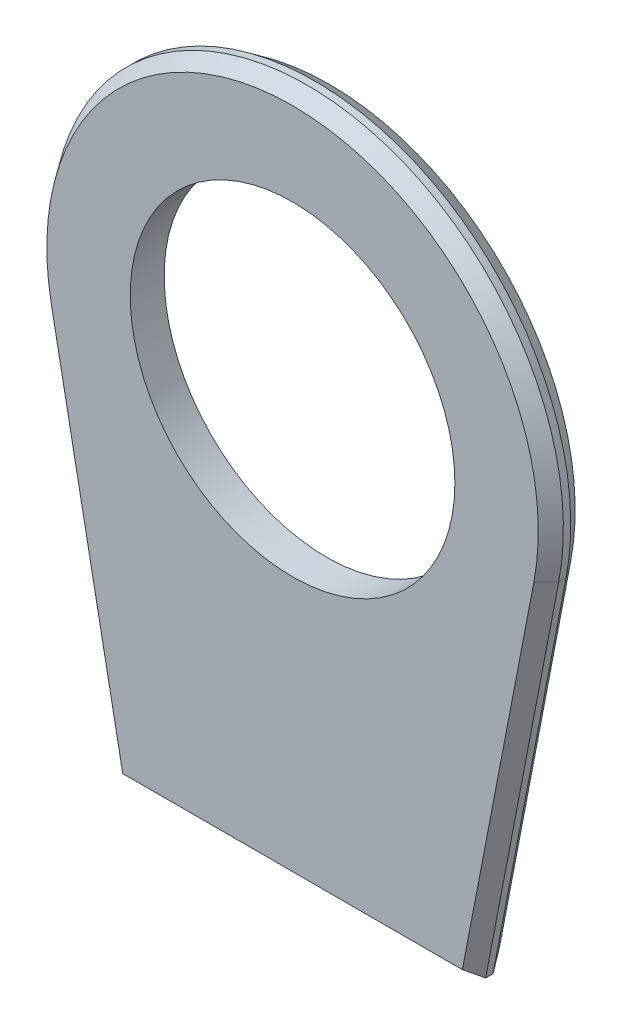
SolidWorks part; units mm, degrees
ref_plane "Front Plane" through (0, 0, 0) normal (0, 0, 1) x (1, 0, 0)
ref_plane "Top Plane" through (0, 0, 0) normal (0, 1, 0) x (1, 0, 0)
ref_plane "Right Plane" through (0, 0, 0) normal (1, 0, 0) x (0, 0, -1)
sketch "Sketch1" plane through (0, 0, 0) normal (0, 0, 1) x (1, 0, 0)
  line L0 (0, -94.8031) -> (0, 121.5186) construction
  line L1 (-120.85, 0) -> (120.85, 0)
  line L2 (120.85, 0) -> (170.3708, 257.1967)
  line L3 (-120.85, 0) -> (-170.3708, 257.1967)
  arc A0 (170.3708, 257.1967) -> (-170.3708, 257.1967) centre (0, 290) ccw
  circle A1 centre (0, 290) radius 110
  dimension "D1" = 347
  dimension "D5" = 220
  dimension "D2" = 290
  dimension "D3" = 241.7
  dimension "D4" = 241.7
extrude "Boss-Extrude1" add sketch "Sketch1" along normal blind 25
sketch "Sketch2" plane through (0, 0, 0) normal (0, 0, 1) x (1, 0, 0)
  circle A0 centre (0, 290) radius 110 construction
  circle A1 centre (0, 290) radius 110
  circle A2 centre (0, 290) radius 123
  dimension "D1" = 246
extrude "Cut-Extrude2" cut sketch "Sketch2" along normal blind 2
chamfer "Chamfer1" distance 7 distance2 10 4 edges at (145.6104, 128.5984, 0) (0, 463.5, 0) (-145.6104, 128.5984, 0) (0, 0, 0)
chamfer "Chamfer2" distance 10 distance2 7 4 edges at (145.6104, 128.5984, 25) (0, 463.5, 25) (-145.6104, 128.5984, 25) (0, 0, 25)
